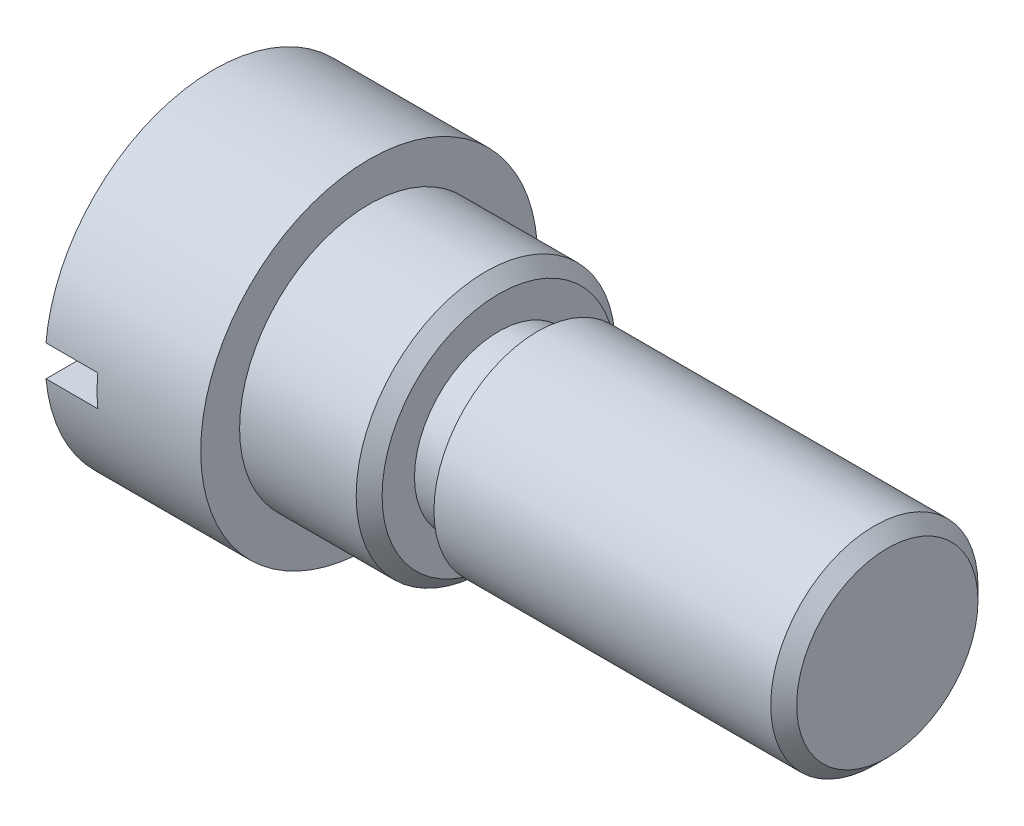
SolidWorks part; units mm, degrees
material "45#"
ref_plane "Front" through (0, 0, 0) normal (0, 0, 1) x (1, 0, 0)
ref_plane "Top" through (0, 0, 0) normal (0, 1, 0) x (1, 0, 0)
ref_plane "Right" through (0, 0, 0) normal (1, 0, 0) x (0, 0, -1)
sketch "草图2" plane through (0, 0, 0) normal (1, 0, 0) x (0, 0, -1)
  circle A0 centre (0, 0) radius 5
  dimension "D1" = 10
extrude "凸台-拉伸1" add sketch "草图2" along normal blind 5
sketch "草图5" plane through (0, 0, 0) normal (-1, 0, 0) x (0, 0, 1)
  circle A0 centre (0, 0) radius 6.5
  dimension "D1" = 13
extrude "凸台-拉伸2" add sketch "草图5" along normal blind 6
sketch "草图6" plane through (-6, 0, 0) normal (-1, 0, 0) x (0, 0, 1)
  line L1 (-15, 0.6) -> (15, 0.6)
  line L2 (-15, 0.6) -> (-15, -0.6)
  line L3 (-15, -0.6) -> (15, -0.6)
  line L4 (15, 0.6) -> (15, -0.6)
  line L5 (-15, 0.6) -> (15, -0.6) construction
  line L6 (-15, -0.6) -> (15, 0.6) construction
  point P0 (0, 0)
  dimension "D1" = 1.2
  dimension "D2" = 30
extrude "切除-拉伸1" cut sketch "草图6" against normal blind 2
sketch "草图7" plane through (5, 0, 0) normal (1, 0, 0) x (0, 0, -1)
  circle A0 centre (0, 0) radius 4
  dimension "D1" = 8
extrude "凸台-拉伸3" add sketch "草图7" along normal blind 15
cosmetic thread "装饰螺纹线1" parameters "D1"=13.5, "D2"=6.647
chamfer "倒角3" distance 0.5 angle 45 2 edges at (20, 0, -4) (5, 0, -5)
sketch "草图8" plane through (0, 0, 0) normal (0, 1, 0) x (1, 0, 0)
  line L0 (0, 0) -> (17.4631, 0) construction
  line L1 (5, -5) -> (5, 5) construction
  line L2 (5, 3.25) -> (6.5, 3.25)
  line L3 (5, 3.25) -> (5, 5.0449)
  line L4 (5, 5.0449) -> (6.5, 5.0449)
  line L5 (6.5, 3.25) -> (6.5, 5.0449)
  dimension "D1" = 6.5
  dimension "D2" = 1.5
revolve "切除-旋转1" cut sketch "草图8" angle 360 about L0
